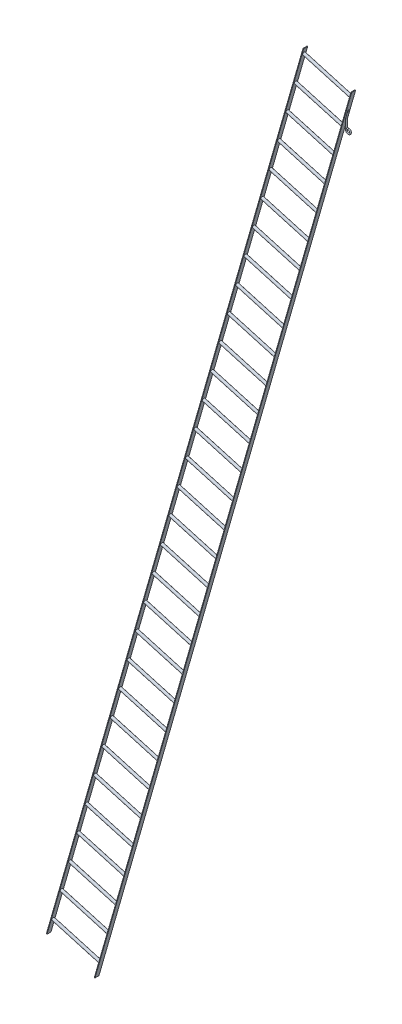
from build123d import *

# Parameters (mm, degrees)
SWEEP2_PROFILE_R                               = 6
CHAMFER1_SIZE                                  = 0.5
SKETCH1_W                                      = 40
SKETCH1_H                                      = 6
GB_T_704_1988_HOT_ROLLED_FLAT_STEEL_40_6_DEPTH = 9210
SKETCH1_ON_SEGMENT_2_W                         = 40
SKETCH1_ON_SEGMENT_2_H                         = 6
GB_T_704_1988_HOT_ROLLED_FLAT_STEEL_2_DEPTH    = 9210
SKETCH13_R                                     = 13.4
SKETCH13_R_2                                   = 10.4
GB_T_6728_2002_ROUND_TUBE_26_8_X_3_2_DEPTH     = 494
SKETCH13_ON_SEGMENT_2_R                        = 13.4
SKETCH13_ON_SEGMENT_2_R_2                      = 10.4
GB_T_6728_2002_ROUND_TUBE_26_8_X_3_2_2_DEPTH   = 494
LPATTERN1_COUNT                                = 30
LPATTERN1_PITCH                                = 300


with BuildPart() as part:
    # Sweep2: sweep along a path in 18 (ProfileFeature) (+7 more in 7 files) Sketch1
    with BuildLine(Plane.XY) as sweep2_path:
        Line((2.366140089, 179), (-19.767570176, 101.810579127))
        ThreePointArc((-19.767570176, 101.810579127), (-19.941608412, 100.991793598), (-20, 100.156754992))
        Line((-20, 100.156754992), (-20, 0))
        ThreePointArc((-20, 0), (14.142135624, -14.142135624), (0, 20))
        Line((0, 20), (-13.95, 20))
    # Sweep2 profile (on start of the path) → Sweep2 (sweep)
    with BuildSketch(Plane(origin=(2.366140089, 179, 0), x_dir=(-0.9612616959383187, 0.27563735581700005, 0), z_dir=(-0.27563735581700005, -0.9612616959383187, 0))):
        Circle(SWEEP2_PROFILE_R)
    sweep(path=sweep2_path.line)

    # Chamfer1
    chamfer1_edges = [part.edges().sort_by_distance(p)[0] for p in [
        (8.133710265, 177.346175865, 0),
    ]]
    chamfer(chamfer1_edges, length=CHAMFER1_SIZE)


with BuildPart() as body_2:
    # Sketch1 → GB/T 704-1988 hot-rolled flat steel 40×6(1) (new body)
    with BuildSketch(Plane(origin=(-2488.272192777, -8485.120364749, -20), x_dir=(0, 0, 1), z_dir=(-0.2756373558169933, -0.9612616959383207, 0))):
        with Locations((20, 3)):
            Rectangle(SKETCH1_W, SKETCH1_H)
    extrude(amount=-GB_T_704_1988_HOT_ROLLED_FLAT_STEEL_40_6_DEPTH)


with BuildPart() as body_3:
    # Sketch1 on segment 2 (carried to segment 2) → GB_T 704-1988 hot-rolled flat steel  2 (new body)
    with BuildSketch(Plane(origin=(-424.515423496, 504.264708616, -20), x_dir=(0, 0, 1), z_dir=(-0.275637356, -0.961261696, 0))):
        with Locations((20, 3)):
            Rectangle(SKETCH1_ON_SEGMENT_2_W, SKETCH1_ON_SEGMENT_2_H)
    extrude(amount=GB_T_704_1988_HOT_ROLLED_FLAT_STEEL_2_DEPTH)


with BuildPart() as body_4:
    # Sketch13 → GB/T 6728-2002 round tube 26.8 X 3(2) (new body)
    with BuildSketch(Plane(origin=(-2921.789867198, -8204.766256585, 0), x_dir=(0.2756373558170012, 0.9612616959383185, 0), z_dir=(0.9612616959383185, -0.2756373558170012, 0))):
        Circle(SKETCH13_R)
        Circle(SKETCH13_R_2, mode=Mode.SUBTRACT)
    extrude(amount=GB_T_6728_2002_ROUND_TUBE_26_8_X_3_2_DEPTH)

    # Trim_Extend1 15
    split(bisect_by=Plane(origin=(-56.776544157, 16.280412056, 0), x_dir=(-0.275637356, -0.961261696, 0), z_dir=(-0.961261696, 0.275637356, 0)), keep=Keep.TOP)


with BuildPart() as body_5:
    # Sketch13 on segment 2 (carried to segment 2) → GB_T 6728-2002 round tube 26.8 X 3_2 2 (new body)
    with BuildSketch(Plane(origin=(-2839.098660453, -7916.387747803, 0), x_dir=(0.275637356, 0.961261696, 0), z_dir=(0.961261696, -0.275637356, 0))):
        Circle(SKETCH13_ON_SEGMENT_2_R)
        Circle(SKETCH13_ON_SEGMENT_2_R_2, mode=Mode.SUBTRACT)
    extrude(amount=GB_T_6728_2002_ROUND_TUBE_26_8_X_3_2_2_DEPTH)

    # Trim_Extend1 17: cut body 2
    add(body_2.part, mode=Mode.SUBTRACT)


with BuildPart() as lpattern1_1:
    # LPattern1: pattern copy
    add(body_5.part.moved(Location(Vector(0.27563735581699933, 0.9612616959383189, 0) * (1 * LPATTERN1_PITCH))))


with BuildPart() as lpattern1_2:
    # LPattern1: pattern copy
    add(body_5.part.moved(Location(Vector(0.27563735581699933, 0.9612616959383189, 0) * (2 * LPATTERN1_PITCH))))


with BuildPart() as lpattern1_3:
    # LPattern1: pattern copy
    add(body_5.part.moved(Location(Vector(0.27563735581699933, 0.9612616959383189, 0) * (3 * LPATTERN1_PITCH))))


with BuildPart() as lpattern1_4:
    # LPattern1: pattern copy
    add(body_5.part.moved(Location(Vector(0.27563735581699933, 0.9612616959383189, 0) * (4 * LPATTERN1_PITCH))))


with BuildPart() as lpattern1_5:
    # LPattern1: pattern copy
    add(body_5.part.moved(Location(Vector(0.27563735581699933, 0.9612616959383189, 0) * (5 * LPATTERN1_PITCH))))


with BuildPart() as lpattern1_6:
    # LPattern1: pattern copy
    add(body_5.part.moved(Location(Vector(0.27563735581699933, 0.9612616959383189, 0) * (6 * LPATTERN1_PITCH))))


with BuildPart() as lpattern1_7:
    # LPattern1: pattern copy
    add(body_5.part.moved(Location(Vector(0.27563735581699933, 0.9612616959383189, 0) * (7 * LPATTERN1_PITCH))))


with BuildPart() as lpattern1_8:
    # LPattern1: pattern copy
    add(body_5.part.moved(Location(Vector(0.27563735581699933, 0.9612616959383189, 0) * (8 * LPATTERN1_PITCH))))


with BuildPart() as lpattern1_9:
    # LPattern1: pattern copy
    add(body_5.part.moved(Location(Vector(0.27563735581699933, 0.9612616959383189, 0) * (9 * LPATTERN1_PITCH))))


with BuildPart() as lpattern1_10:
    # LPattern1: pattern copy
    add(body_5.part.moved(Location(Vector(0.27563735581699933, 0.9612616959383189, 0) * (10 * LPATTERN1_PITCH))))


with BuildPart() as lpattern1_11:
    # LPattern1: pattern copy
    add(body_5.part.moved(Location(Vector(0.27563735581699933, 0.9612616959383189, 0) * (11 * LPATTERN1_PITCH))))


with BuildPart() as lpattern1_12:
    # LPattern1: pattern copy
    add(body_5.part.moved(Location(Vector(0.27563735581699933, 0.9612616959383189, 0) * (12 * LPATTERN1_PITCH))))


with BuildPart() as lpattern1_13:
    # LPattern1: pattern copy
    add(body_5.part.moved(Location(Vector(0.27563735581699933, 0.9612616959383189, 0) * (13 * LPATTERN1_PITCH))))


with BuildPart() as lpattern1_14:
    # LPattern1: pattern copy
    add(body_5.part.moved(Location(Vector(0.27563735581699933, 0.9612616959383189, 0) * (14 * LPATTERN1_PITCH))))


with BuildPart() as lpattern1_15:
    # LPattern1: pattern copy
    add(body_5.part.moved(Location(Vector(0.27563735581699933, 0.9612616959383189, 0) * (15 * LPATTERN1_PITCH))))


with BuildPart() as lpattern1_16:
    # LPattern1: pattern copy
    add(body_5.part.moved(Location(Vector(0.27563735581699933, 0.9612616959383189, 0) * (16 * LPATTERN1_PITCH))))


with BuildPart() as lpattern1_17:
    # LPattern1: pattern copy
    add(body_5.part.moved(Location(Vector(0.27563735581699933, 0.9612616959383189, 0) * (17 * LPATTERN1_PITCH))))


with BuildPart() as lpattern1_18:
    # LPattern1: pattern copy
    add(body_5.part.moved(Location(Vector(0.27563735581699933, 0.9612616959383189, 0) * (18 * LPATTERN1_PITCH))))


with BuildPart() as lpattern1_19:
    # LPattern1: pattern copy
    add(body_5.part.moved(Location(Vector(0.27563735581699933, 0.9612616959383189, 0) * (19 * LPATTERN1_PITCH))))


with BuildPart() as lpattern1_20:
    # LPattern1: pattern copy
    add(body_5.part.moved(Location(Vector(0.27563735581699933, 0.9612616959383189, 0) * (20 * LPATTERN1_PITCH))))


with BuildPart() as lpattern1_21:
    # LPattern1: pattern copy
    add(body_5.part.moved(Location(Vector(0.27563735581699933, 0.9612616959383189, 0) * (21 * LPATTERN1_PITCH))))


with BuildPart() as lpattern1_22:
    # LPattern1: pattern copy
    add(body_5.part.moved(Location(Vector(0.27563735581699933, 0.9612616959383189, 0) * (22 * LPATTERN1_PITCH))))


with BuildPart() as lpattern1_23:
    # LPattern1: pattern copy
    add(body_5.part.moved(Location(Vector(0.27563735581699933, 0.9612616959383189, 0) * (23 * LPATTERN1_PITCH))))


with BuildPart() as lpattern1_24:
    # LPattern1: pattern copy
    add(body_5.part.moved(Location(Vector(0.27563735581699933, 0.9612616959383189, 0) * (24 * LPATTERN1_PITCH))))


with BuildPart() as lpattern1_25:
    # LPattern1: pattern copy
    add(body_5.part.moved(Location(Vector(0.27563735581699933, 0.9612616959383189, 0) * (25 * LPATTERN1_PITCH))))


with BuildPart() as lpattern1_26:
    # LPattern1: pattern copy
    add(body_5.part.moved(Location(Vector(0.27563735581699933, 0.9612616959383189, 0) * (26 * LPATTERN1_PITCH))))


with BuildPart() as lpattern1_27:
    # LPattern1: pattern copy
    add(body_5.part.moved(Location(Vector(0.27563735581699933, 0.9612616959383189, 0) * (27 * LPATTERN1_PITCH))))


with BuildPart() as lpattern1_28:
    # LPattern1: pattern copy
    add(body_5.part.moved(Location(Vector(0.27563735581699933, 0.9612616959383189, 0) * (28 * LPATTERN1_PITCH))))


with BuildPart() as lpattern1_29:
    # LPattern1: pattern copy
    add(body_5.part.moved(Location(Vector(0.27563735581699933, 0.9612616959383189, 0) * (29 * LPATTERN1_PITCH))))


solid = Compound([part.part, body_2.part, body_3.part, body_4.part, body_5.part, lpattern1_1.part, lpattern1_2.part, lpattern1_3.part, lpattern1_4.part, lpattern1_5.part, lpattern1_6.part, lpattern1_7.part, lpattern1_8.part, lpattern1_9.part, lpattern1_10.part, lpattern1_11.part, lpattern1_12.part, lpattern1_13.part, lpattern1_14.part, lpattern1_15.part, lpattern1_16.part, lpattern1_17.part, lpattern1_18.part, lpattern1_19.part, lpattern1_20.part, lpattern1_21.part, lpattern1_22.part, lpattern1_23.part, lpattern1_24.part, lpattern1_25.part, lpattern1_26.part, lpattern1_27.part, lpattern1_28.part, lpattern1_29.part])
